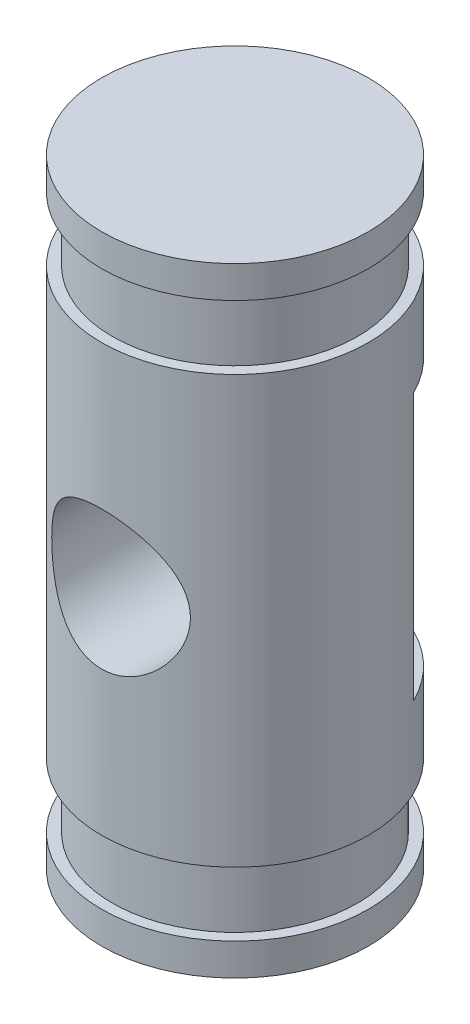
SolidWorks part; units mm, degrees
ref_plane "Front Plane" through (0, 0, 0) normal (0, 0, 1) x (1, 0, 0)
ref_plane "Top Plane" through (0, 0, 0) normal (0, 1, 0) x (1, 0, 0)
ref_plane "Right Plane" through (0, 0, 0) normal (1, 0, 0) x (0, 0, -1)
sketch "Sketch1" plane through (0, 0, 0) normal (0, 1, 0) x (1, 0, 0)
  circle A0 centre (0, 0) radius 12.5
  dimension "D1" = 25
extrude "Boss-Extrude1" add sketch "Sketch1" along normal mid plane 58
sketch "Sketch2" plane through (0, 29, 0) normal (0, 1, 0) x (1, 0, 0)
  circle A0 centre (0, 0) radius 11.5
  circle A1 centre (0, 0) radius 12.5
  dimension "D1" = 23
extrude "Cut-Extrude1" cut sketch "Sketch2" against normal blind 6 from offset 3 offset against normal yes
mirror "Mirror1" about plane through (0, 0, 0) normal (0, 1, 0) of "Cut-Extrude1"
sketch "Sketch3" plane through (0, 0, 0) normal (1, 0, 0) x (0, 0, -1)
  line L0 (0, 0) -> (8.7632, 0) construction
  line L1 (12.5, -20) -> (12.5, 20) construction
  line L2 (12.5, 12.5) -> (5.5, 12.5)
  line L3 (12.5, 12.5) -> (12.5, -12.5)
  line L4 (12.5, -12.5) -> (5.5, -12.5)
  line L5 (5.5, 12.5) -> (5.5, -12.5)
  dimension "D1" = 7
  dimension "D2" = 25
extrude "Cut-Extrude2" cut sketch "Sketch3" against normal mid plane 66
sketch "Sketch4" plane through (0, 0, -5.5) normal (0, 0, -1) x (-1, 0, 0)
  circle A0 centre (0, 0) radius 6.5
  dimension "D1" = 13
extrude "Cut-Extrude3" cut sketch "Sketch4" against normal through all
